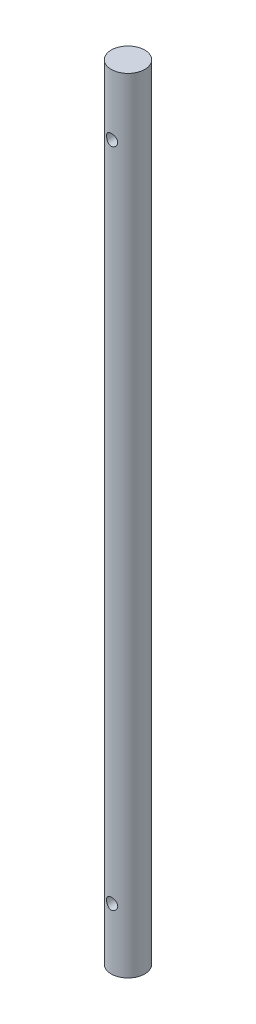
from build123d import *

# Parameters (mm, degrees)
SKETCH_1_R          = 6
EXTRUDE_1_DEPTH     = 140
SKETCH_3_R          = 2
CUT_EXTRUDE_1_DEPTH = 60


with BuildPart() as part:
    # 草图1 → 凸台-拉伸1 (new, symmetric)
    with BuildSketch(Plane(origin=(0, 0, 0), x_dir=(1, 0, 0), z_dir=(0, 1, 0))):
        with Locations(Location((0, 0, 0), (0, 0, 270))):
            Circle(SKETCH_1_R)
    extrude(amount=EXTRUDE_1_DEPTH, both=True)

    # 草图3 → 切除-拉伸1 (cut)
    with BuildSketch(Plane.XY.offset(11)):
        with Locations(Location((0, -118.208062, 0), (0, 0, 89.999999987))):
            Circle(SKETCH_3_R)
    cut_extrude_1 = extrude(amount=-CUT_EXTRUDE_1_DEPTH, mode=Mode.SUBTRACT)

    # 镜向1: 切除-拉伸1 across plane
    add(cut_extrude_1.mirror(Plane.ZX), mode=Mode.SUBTRACT)


solid = part.part
